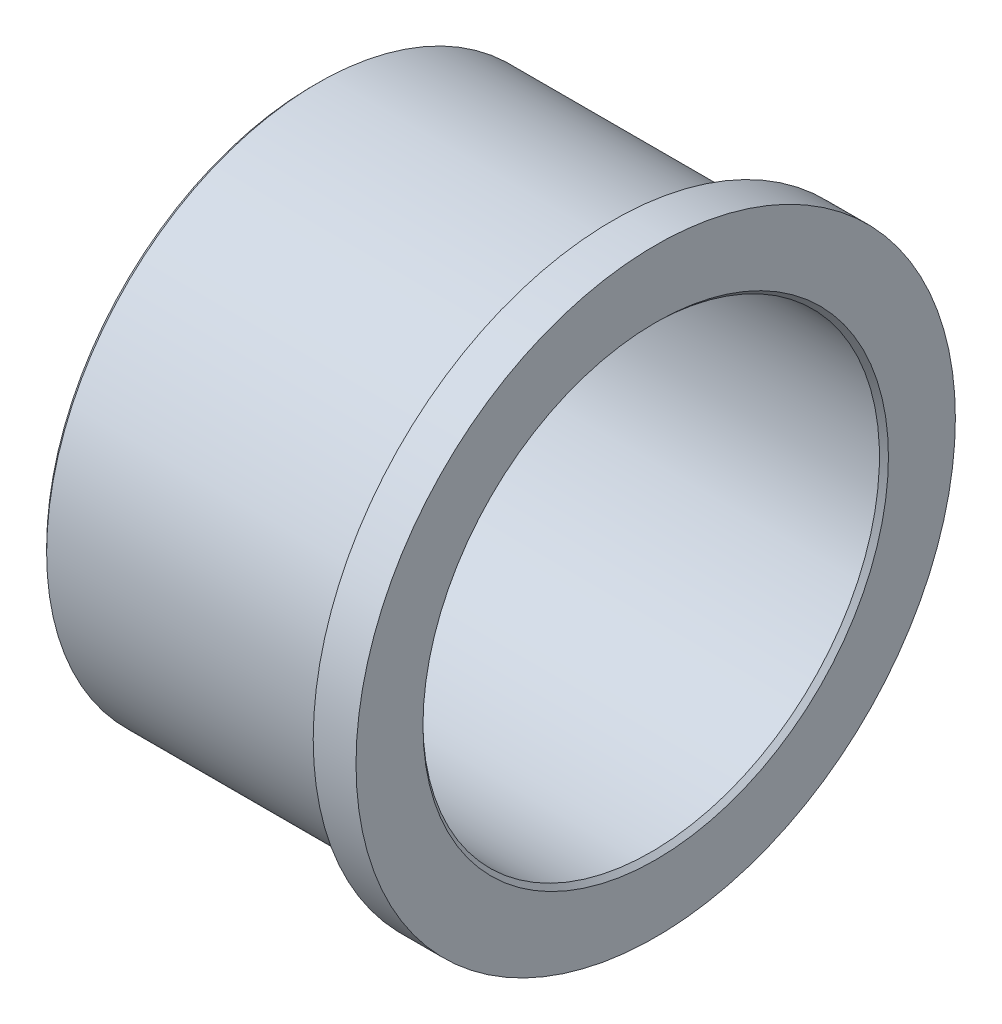
SolidWorks part; units mm, degrees
material "黄铜"
ref_plane "前视基准面" through (0, 0, 0) normal (0, 0, 1) x (1, 0, 0)
ref_plane "上视基准面" through (0, 0, 0) normal (0, 1, 0) x (1, 0, 0)
ref_plane "右视基准面" through (0, 0, 0) normal (1, 0, 0) x (0, 0, -1)
sketch "尺寸草图" plane through (0, 0, 0) normal (0, 0, 1) x (1, 0, 0)
  line L0 (-30, 0) -> (30, 0) construction
  line L1 (0, 0) -> (0, 40) construction
  line L2 (-30, 40.7726) -> (-29.2, 40)
  line L3 (-29.2, 40) -> (29.2, 40)
  line L4 (29.2, 40) -> (30, 40.7726)
  line L5 (30, 40.7726) -> (30, 52.5)
  line L6 (30, 52.5) -> (22.5, 52.5)
  line L7 (22.5, 52.5) -> (22.5, 47.3)
  line L8 (22.5, 47.3) -> (20.5, 47.3)
  line L9 (20.5, 47.3) -> (20.5, 47.5)
  line L10 (20.5, 47.5) -> (-29.2, 47.5)
  line L11 (-29.2, 47.5) -> (-30, 46.7)
  line L12 (-30, 46.7) -> (-30, 40.7726)
  dimension "D1" = 44
  dimension "内径d1" = 80
  dimension "倒角C1" = 0.8
  dimension "D2" = 0.2
  dimension "外径d2" = 95
  dimension "翻边外径d3" = 105
  dimension "宽度b1" = 60
  dimension "翻边宽度b2" = 7.5
  dimension "退刀槽宽度u" = 2
  dimension "倒角C2" = 0.8
  dimension "C2角度" = 45
revolve "旋转1" add sketch "尺寸草图" angle 360 about L0
